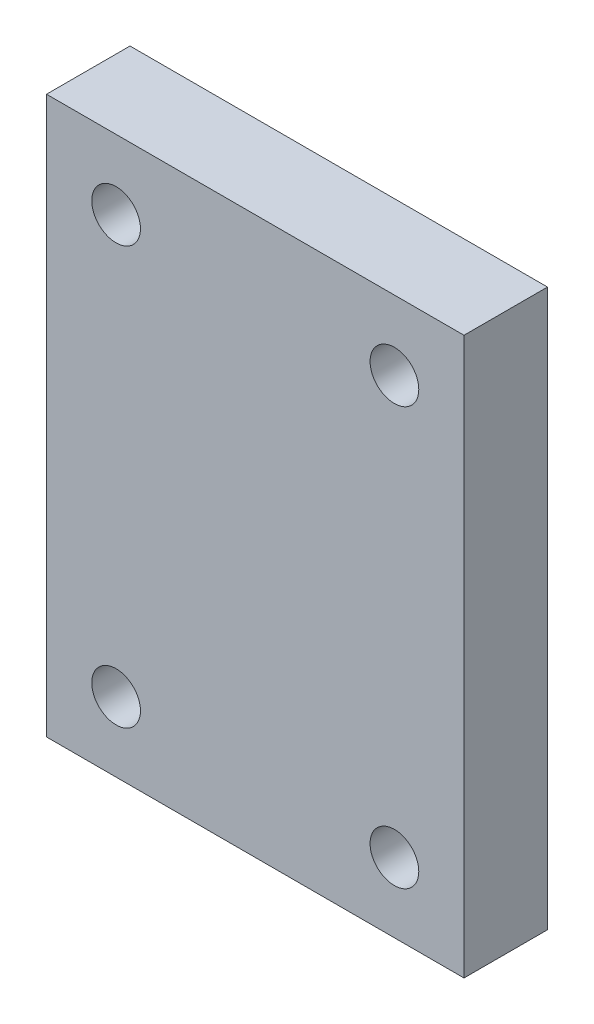
SolidWorks part; units mm, degrees
material "Q235"
ref_plane "Front Plane" through (0, 0, 0) normal (0, 0, 1) x (1, 0, 0)
ref_plane "Top Plane" through (0, 0, 0) normal (0, 1, 0) x (1, 0, 0)
ref_plane "Right Plane" through (0, 0, 0) normal (1, 0, 0) x (0, 0, -1)
sketch "Sketch1" plane through (0, 0, 0) normal (0, 0, 1) x (1, 0, 0)
  line L1 (0, 0) -> (150, 0)
  line L2 (0, 0) -> (0, 200)
  line L3 (0, 200) -> (150, 200)
  line L4 (150, 0) -> (150, 200)
  dimension "D1" = 150
  dimension "D2" = 200
extrude "Boss-Extrude1" add sketch "Sketch1" along normal blind 30
hole_wizard "M20 Threaded hole1" positions "3DSketch1" profile "Sketch2" tap size "M20" standard "GB" end condition through all
sketch3d "3DSketch1"
  line L0 (0, 200, 30) -> (0, 0, 30) construction
  line L1 (150, 200, 30) -> (0, 200, 30) construction
  point P0 (25, 175, 30)
  point P2 (125, 175, 30)
  point P4 (25, 25, 30)
  point P6 (125, 25, 30)
  dimension "D1" = 100
  dimension "D2" = 25
  dimension "D3" = 150
  dimension "D4" = 25
sketch "Sketch2" plane through (25, 175, 30) normal (1, 0, 0) x (0, -1, 0)
  line L0 (0, 0) -> (0, 30)
  line L1 (0, 30) -> (8.75, 30)
  line L2 (8.75, 30) -> (8.75, 0)
  line L5 (8.75, 0) -> (0, 0)
  line L11 (0, -6.35) -> (0, 107.95) construction
  dimension "通孔螺纹孔钻头直径" = 17.5
  dimension "通孔螺纹孔钻头深度" = 30
cosmetic thread "孔螺蚊线1"
cosmetic thread "孔螺蚊线2"
cosmetic thread "孔螺蚊线3"
cosmetic thread "孔螺蚊线4"
sketch "Sketch3" plane through (0, 0, 30) normal (0, 0, 1) x (1, 0, 0)
  line L0 (75, 200) -> (75, 0) construction
  line L1 (150, 200) -> (0, 200) construction
  line L2 (0, 0) -> (150, 0) construction
  line L3 (0, 100) -> (150, 100) construction
  line L4 (0, 200) -> (0, 0) construction
  line L5 (150, 0) -> (150, 200) construction
